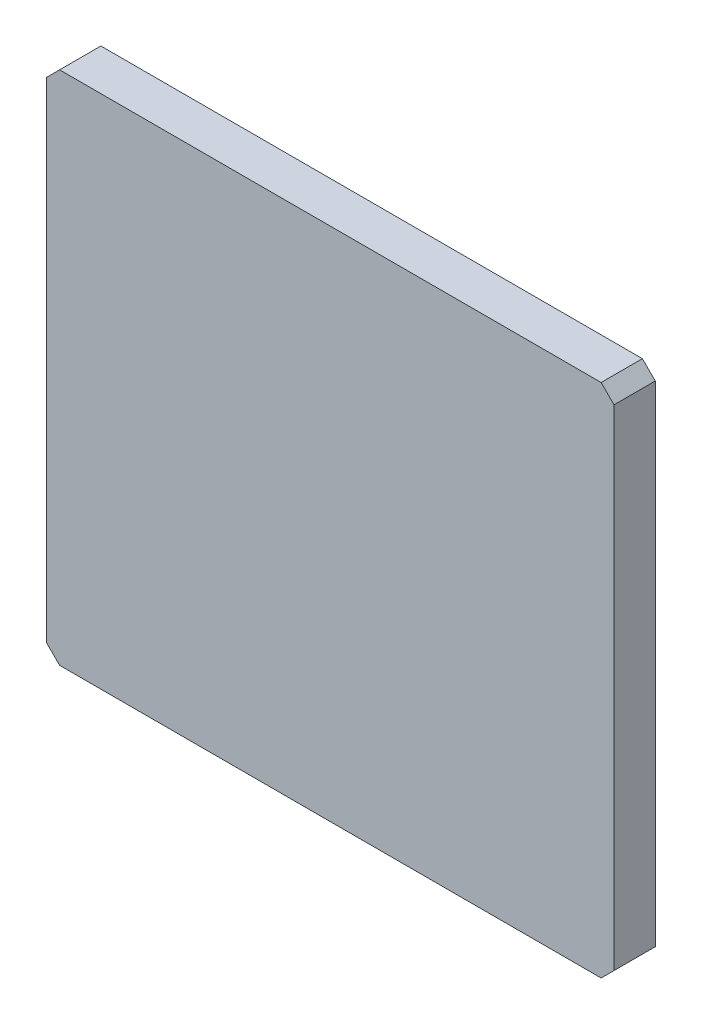
SolidWorks part; units mm, degrees
material "Q235-A "
ref_plane "前视基准面" through (0, 0, 0) normal (0, 0, 1) x (1, 0, 0)
ref_plane "上视基准面" through (0, 0, 0) normal (0, 1, 0) x (1, 0, 0)
ref_plane "右视基准面" through (0, 0, 0) normal (1, 0, 0) x (0, 0, -1)
sketch "草图1" plane through (0, 0, 0) normal (0, 0, 1) x (1, 0, 0)
  line L1 (0, 0) -> (220, 0)
  line L2 (0, 0) -> (0, -200)
  line L3 (0, -200) -> (220, -200)
  line L4 (220, 0) -> (220, -200)
  dimension "D1" = 200
  dimension "D2" = 220
extrude "凸台-拉伸1" add sketch "草图1" along normal blind 16
sketch "草图2" plane through (0, 0, 16) normal (0, 0, 1) x (1, 0, 0)
  line L0 (0, -100) -> (220, -100) construction
  line L1 (0, 0) -> (0, -200) construction
  line L2 (220, -200) -> (220, 0) construction
  line L3 (110, -55) -> (110, -100) construction
  line L4 (50, -55) -> (170, -55) construction
  line L5 (50, -55) -> (50, -145) construction
  line L6 (50, -145) -> (170, -145) construction
  line L7 (170, -55) -> (170, -145) construction
  line L8 (50, -55) -> (170, -145) construction
  line L9 (50, -145) -> (170, -55) construction
  line L10 (29.75, -119.75) -> (70.25, -170.25) construction
  line L11 (34.75, -29.75) -> (65.25, -29.75)
  line L12 (29.75, -34.75) -> (29.75, -75.25)
  line L13 (34.75, -80.25) -> (65.25, -80.25)
  line L14 (70.25, -34.75) -> (70.25, -75.25)
  line L15 (29.75, -29.75) -> (70.25, -80.25) construction
  line L16 (29.75, -80.25) -> (70.25, -29.75) construction
  line L17 (29.75, -170.25) -> (70.25, -119.75) construction
  line L18 (70.25, -165.25) -> (70.25, -124.75)
  line L19 (34.75, -119.75) -> (65.25, -119.75)
  line L20 (29.75, -165.25) -> (29.75, -124.75)
  line L21 (34.75, -170.25) -> (65.25, -170.25)
  line L22 (190.25, -170.25) -> (149.75, -119.75) construction
  line L23 (190.25, -80.25) -> (149.75, -29.75) construction
  line L24 (190.25, -29.75) -> (149.75, -80.25) construction
  line L25 (190.25, -119.75) -> (149.75, -170.25) construction
  line L26 (170, -55) -> (170, -145) construction
  line L27 (185.25, -170.25) -> (154.75, -170.25)
  line L28 (190.25, -165.25) -> (190.25, -124.75)
  line L29 (185.25, -119.75) -> (154.75, -119.75)
  line L30 (149.75, -165.25) -> (149.75, -124.75)
  line L31 (149.75, -34.75) -> (149.75, -75.25)
  line L32 (185.25, -80.25) -> (154.75, -80.25)
  line L33 (190.25, -34.75) -> (190.25, -75.25)
  line L34 (185.25, -29.75) -> (154.75, -29.75)
  circle A0 centre (50, -55) radius 20 construction
  circle A1 centre (50, -145) radius 20 construction
  circle A2 centre (170, -145) radius 20 construction
  circle A3 centre (170, -55) radius 20 construction
  arc A4 (70.25, -75.25) -> (65.25, -80.25) centre (65.25, -75.25) cw
  arc A5 (34.75, -80.25) -> (29.75, -75.25) centre (34.75, -75.25) cw
  arc A6 (70.25, -34.75) -> (65.25, -29.75) centre (65.25, -34.75) ccw
  arc A7 (29.75, -34.75) -> (34.75, -29.75) centre (34.75, -34.75) cw
  circle A8 centre (50, -145) radius 20 construction
  arc A9 (29.75, -165.25) -> (34.75, -170.25) centre (34.75, -165.25) ccw
  arc A10 (70.25, -165.25) -> (65.25, -170.25) centre (65.25, -165.25) cw
  arc A11 (34.75, -119.75) -> (29.75, -124.75) centre (34.75, -124.75) ccw
  arc A12 (70.25, -124.75) -> (65.25, -119.75) centre (65.25, -124.75) ccw
  circle A13 centre (170, -145) radius 20 construction
  circle A14 centre (170, -145) radius 20 construction
  circle A15 centre (170, -55) radius 20 construction
  arc A16 (149.75, -124.75) -> (154.75, -119.75) centre (154.75, -124.75) cw
  arc A17 (185.25, -119.75) -> (190.25, -124.75) centre (185.25, -124.75) cw
  arc A18 (149.75, -165.25) -> (154.75, -170.25) centre (154.75, -165.25) ccw
  arc A19 (190.25, -165.25) -> (185.25, -170.25) centre (185.25, -165.25) cw
  arc A20 (190.25, -34.75) -> (185.25, -29.75) centre (185.25, -34.75) ccw
  arc A21 (149.75, -34.75) -> (154.75, -29.75) centre (154.75, -34.75) cw
  arc A22 (185.25, -80.25) -> (190.25, -75.25) centre (185.25, -75.25) ccw
  arc A23 (149.75, -75.25) -> (154.75, -80.25) centre (154.75, -75.25) ccw
  point P6 (110, -100)
  dimension "D4" = 40
  dimension "D7" = 5
  dimension "D1" = 120
  dimension "D2" = 90
  dimension "D3" = 50
  dimension "D5" = 40.5
  dimension "D6" = 50.5
chamfer "倒角1" distance 5 angle 45 4 edges at (0, -200, 8) (220, -200, 8) (220, 0, 8) (0, 0, 8)
